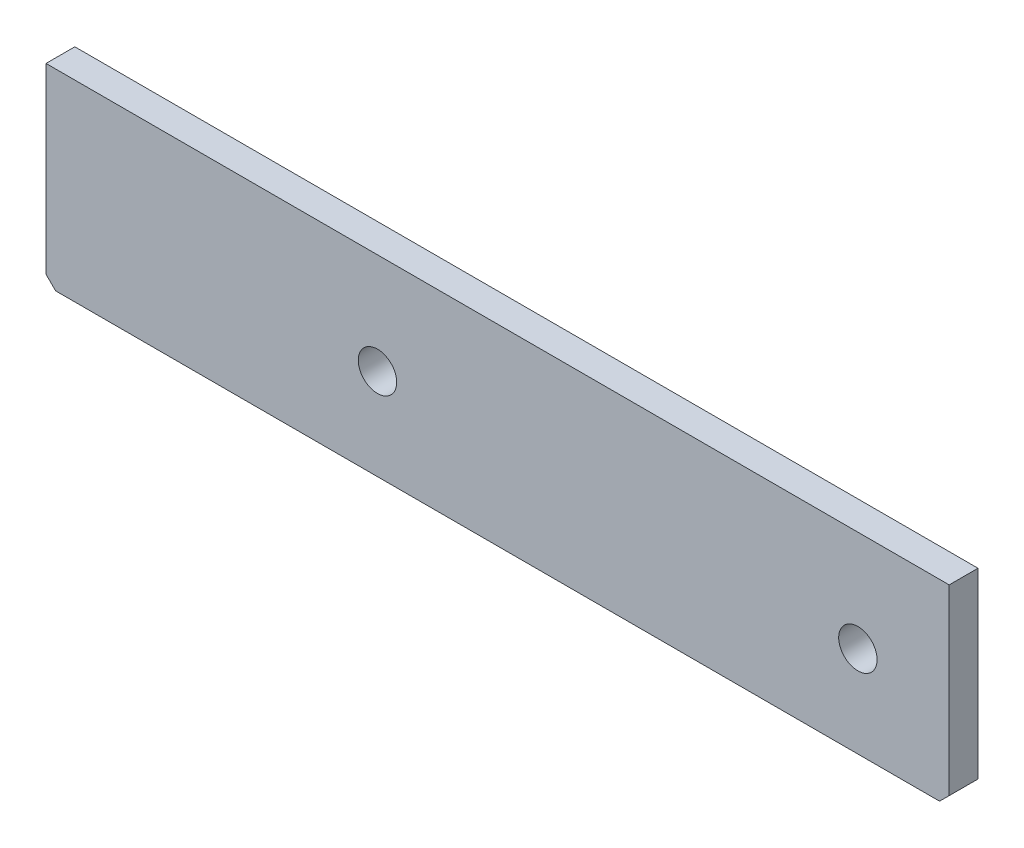
from build123d import *

# Parameters (mm, degrees)
SKETCH1_W           = 188
SKETCH1_H           = 40
BOSS_EXTRUDE1_DEPTH = 6
SKETCH2_R           = 4
CUT_EXTRUDE1_DEPTH  = 6
CHAMFER1_SIZE       = 2


with BuildPart() as part:
    # Sketch1 → Boss-Extrude1 (new body)
    with BuildSketch(Plane.XY):
        Rectangle(SKETCH1_W, SKETCH1_H)
    extrude(amount=BOSS_EXTRUDE1_DEPTH)

    # Sketch2 → Cut-Extrude1 (cut)
    with BuildSketch(Plane.XY.offset(6)):
        with Locations((-25, -1)):
            Circle(SKETCH2_R)
        with Locations((75, -1)):
            Circle(SKETCH2_R)
    extrude(amount=-CUT_EXTRUDE1_DEPTH, mode=Mode.SUBTRACT)

    # Chamfer1
    chamfer1_edges = [part.edges().sort_by_distance(p)[0] for p in [
        (94, -20, 3),
        (-94, -20, 3),
    ]]
    chamfer(chamfer1_edges, length=CHAMFER1_SIZE)


solid = part.part
